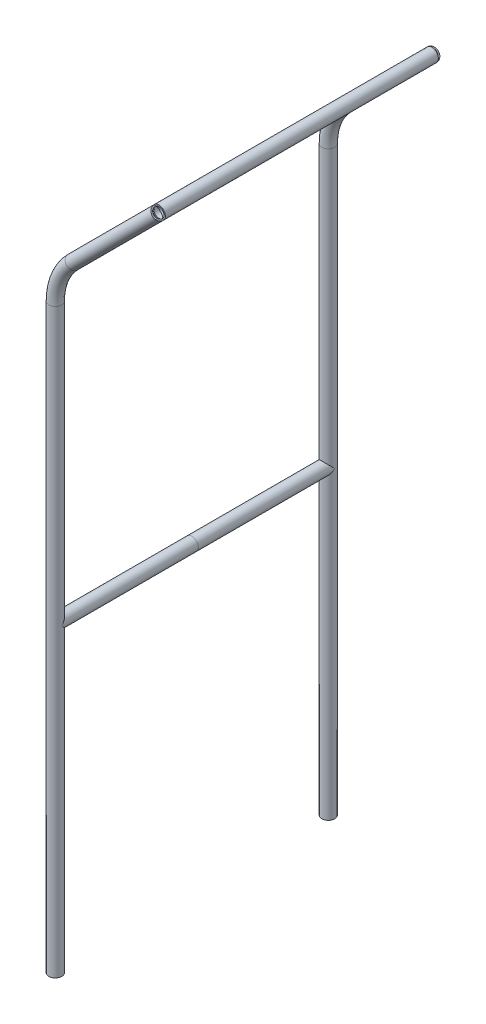
SolidWorks part; units mm, degrees
ref_plane "Front Plane" through (0, 0, 0) normal (0, 0, 1) x (1, 0, 0)
ref_plane "Top Plane" through (0, 0, 0) normal (0, 1, 0) x (1, 0, 0)
ref_plane "Right Plane" through (0, 0, 0) normal (1, 0, 0) x (0, 0, -1)
sketch "草图1" plane through (0, 0, 0) normal (0, 0, 1) x (1, 0, 0)
  line L0 (0, -500) -> (0, 458.5786)
  line L1 (29.2893, 529.2893) -> (170.7107, 670.7107)
  arc A0 (29.2893, 529.2893) -> (0, 458.5786) centre (100, 458.5786) ccw
  point P4 (0, 0)
  dimension "D3" = 200
  dimension "D1" = 200
  dimension "D2" = 135
sketch "Sketch4" plane through (0, 0, 0) normal (1, 0, 0) x (0, 0, -1)
  line L0 (0, 0) -> (-225, 0)
  dimension "D1" = 225
other "Pipe 21.3 X 2.3(1)"
ref_plane "Plane4" through (29.2893, 529.2893, 0) normal (0.7071, 0.7071, 0) x (-0.7071, 0.7071, 0)
sketch "Sketch1" plane through (29.2893, 529.2893, 0) normal (0.7071, 0.7071, 0) x (-0.7071, 0.7071, 0)
  circle A0 centre (0, 0) radius 8.35
  circle A1 centre (0, 0) radius 10.65
  point P3 (0, 0)
  dimension "In_dia" = 16.7
  dimension "Out_dia" = 21.3
other "Pipe 21.3 X 2.3(2)"
ref_plane "Plane5" through (0, 0, 0) normal (0, 0, 1) x (0, -1, 0)
sketch "Sketch11" plane through (0, 0, 0) normal (0, 0, 1) x (0, -1, 0)
  circle A0 centre (0, 0) radius 8.35
  circle A1 centre (0, 0) radius 10.65
  point P3 (0, 0)
  dimension "In_dia" = 16.7
  dimension "Out_dia" = 21.3
mirror "Mirror1" about plane through (0, 0, 225) normal (0, 0, 1) of bodies 103 102 101 104
sketch "Sketch7" plane through (420.7107, 420.7107, 0) normal (0.7071, 0.7071, 0) x (0, 0, -1)
  line L0 (-450, 353.5534) -> (0, 353.5534)
other "Pipe 21.3 X 2.3(3)"
ref_plane "Plane6" through (170.7107, 670.7107, 450) normal (0, 0, -1) x (-0.7071, 0.7071, 0)
sketch "Sketch12" plane through (170.7107, 670.7107, 450) normal (0, 0, -1) x (-0.7071, 0.7071, 0)
  circle A0 centre (0, 0) radius 8.35
  circle A1 centre (0, 0) radius 10.65
  point P3 (0, 0)
  dimension "In_dia" = 16.7
  dimension "Out_dia" = 21.3
